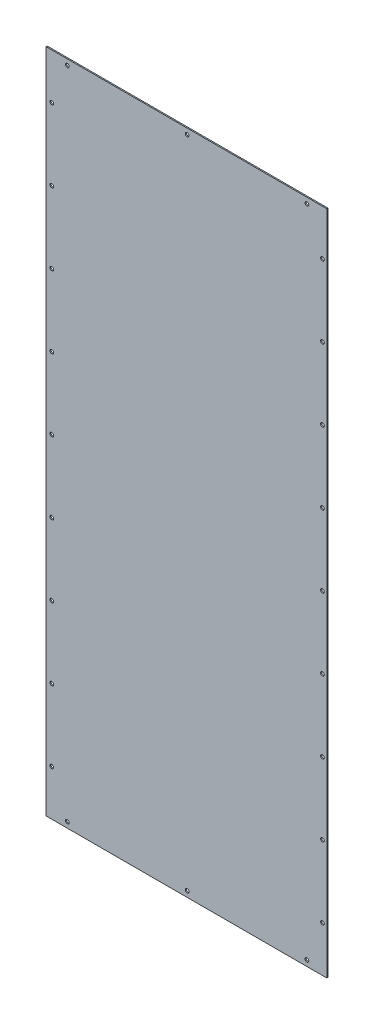
SolidWorks part; units mm, degrees
material "304"
ref_plane "前视基准面" through (0, 0, 0) normal (0, 0, 1) x (1, 0, 0)
ref_plane "上视基准面" through (0, 0, 0) normal (0, 1, 0) x (1, 0, 0)
ref_plane "右视基准面" through (0, 0, 0) normal (1, 0, 0) x (0, 0, -1)
sketch "草图1" plane through (0, 0, 0) normal (0, 0, 1) x (1, 0, 0)
  line L0 (0, 0) -> (451.2544, 0) construction
  line L1 (-247.25, 584) -> (247.25, 584)
  line L2 (-247.25, 584) -> (-247.25, -584)
  line L3 (-247.25, -584) -> (247.25, -584)
  line L4 (247.25, 584) -> (247.25, -584)
  line L5 (-247.25, 584) -> (247.25, -584) construction
  line L6 (-247.25, -584) -> (247.25, 584) construction
  line L7 (0, 0) -> (0, 412.8629) construction
  circle A0 centre (-237.25, 0) radius 3.25
  circle A1 centre (-237.25, -126) radius 3.25
  circle A2 centre (-237.25, -252) radius 3.25
  circle A3 centre (-237.25, -378) radius 3.25
  circle A4 centre (-237.25, -504) radius 3.25
  circle A34 centre (0, -574) radius 3.25
  circle A35 centre (0, 574) radius 3.25
  circle A36 centre (-237.25, 504) radius 3.25
  circle A37 centre (-237.25, 378) radius 3.25
  circle A38 centre (-237.25, 252) radius 3.25
  circle A39 centre (-237.25, 126) radius 3.25
  circle A40 centre (237.25, 126) radius 3.25
  circle A41 centre (237.25, 252) radius 3.25
  circle A42 centre (237.25, 378) radius 3.25
  circle A43 centre (237.25, 504) radius 3.25
  circle A44 centre (237.25, -504) radius 3.25
  circle A45 centre (237.25, -378) radius 3.25
  circle A46 centre (237.25, -252) radius 3.25
  circle A47 centre (237.25, -126) radius 3.25
  circle A48 centre (237.25, 0) radius 3.25
  circle A49 centre (-210, 574) radius 3.25
  circle A50 centre (210, 574) radius 3.25
  circle A51 centre (-210, -574) radius 3.25
  circle A52 centre (210, -574) radius 3.25
  point P0 (0, 0)
  point P49 (0, 0)
  point P50 (0, 0)
  point P51 (0, 0)
  point P56 (120, 441.3004)
  dimension "D3" = 6.5
  dimension "D8" = 420
  dimension "D1" = 494.5
  dimension "D2" = 1168
  dimension "D4" = 10
  dimension "D6" = 10
  dimension "D7" = 80
  dimension "D5" = 5
extrude "凸台-拉伸1" add sketch "草图1" along normal blind 2
sketch "草图2" plane through (0, -584, 0) normal (0, -1, 0) x (1, 0, 0)
  line L0 (-247.25, 2) -> (247.25, 2) construction
  line L1 (247.25, 0) -> (244.75, 0)
  line L2 (247.25, 0) -> (247.25, 2)
  line L3 (247.25, 2) -> (244.75, 2)
  line L4 (244.75, 0) -> (244.75, 2)
  dimension "D1" = 2.5
extrude "切除-拉伸1" cut sketch "草图2" against normal through all
